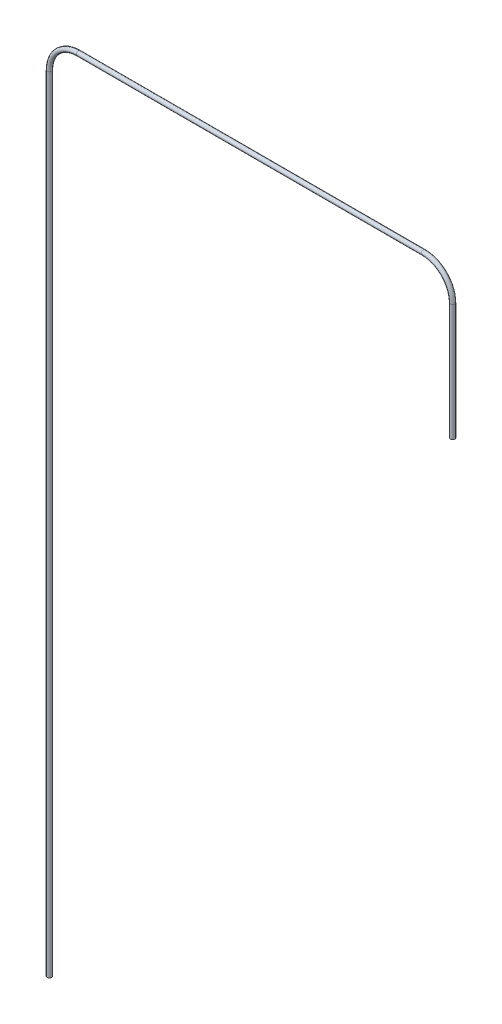
SolidWorks part; units mm, degrees
ref_plane "Front Plane" through (0, 0, 0) normal (0, 0, 1) x (1, 0, 0)
ref_plane "Top Plane" through (0, 0, 0) normal (0, 1, 0) x (1, 0, 0)
ref_plane "Right Plane" through (0, 0, 0) normal (1, 0, 0) x (0, 0, -1)
sketch "Sketch1" plane through (0, 0, 0) normal (0, 0, 1) x (1, 0, 0)
  line L0 (0, 0) -> (0, 1133)
  line L1 (42, 1175) -> (540, 1175)
  line L2 (582, 1133) -> (582, 964.0568)
  arc A0 (540, 1175) -> (582, 1133) centre (540, 1133) cw
  arc A1 (0, 1133) -> (42, 1175) centre (42, 1133) cw
  point P7 (582, 1175)
  point P10 (0, 1175)
  dimension "D3" = 42
  dimension "D1" = 582
  dimension "D2" = 1175
sketch "Sketch2" plane through (0, 0, 0) normal (0, 1, 0) x (1, 0, 0)
  circle A0 centre (0, 0) radius 3.25
  dimension "D1" = 6.5
sweep "Sweep1" add profiles "Sketch2" path "Sketch1"
